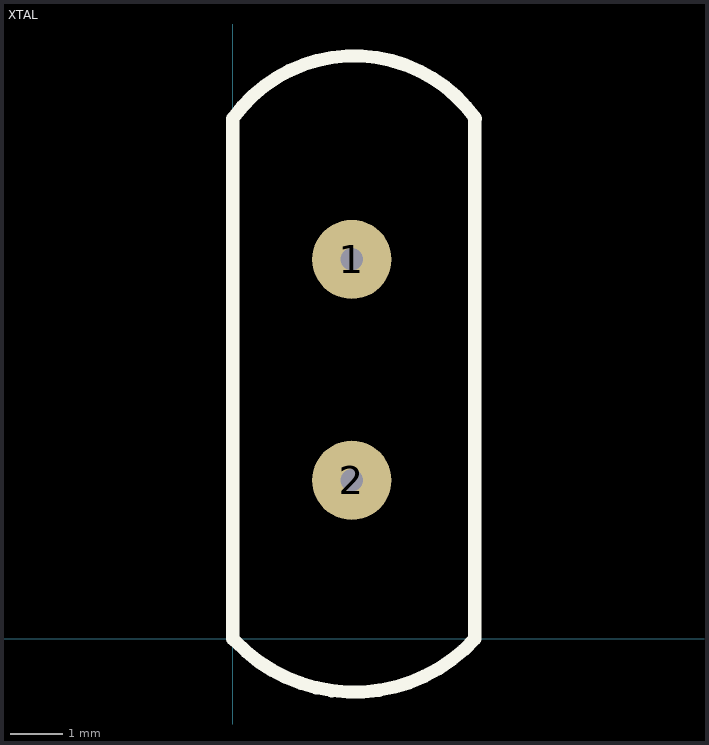
[diagram p0: the footprint, top view; thin cyan lines are the x and y axes]
# Altium footprint library MISC86338-16.PcbLib: 1 footprints
Each footprint in its own frame and in the unit in brackets; x right, y up, seen from the top. Pads: shape width x height; smd on the part's side, far side on the other; paste and mask are expansions set on the pad; w line width, h text height; cw(c..) or ccw(c..) is an arc to the next point about the centre after c.

## XTAL [mil]
pads (2):
  round 60 hole 17.13: 1(90,287.13) 2(90,120)
Top Overlay:
  lines w10: 0,0 0,393.7 cw(c91.77,328.75) 183.68,393.5 ; 1.66,-1.52 ccw(c91.66,83.48) 183.07,0 183.07,393.07